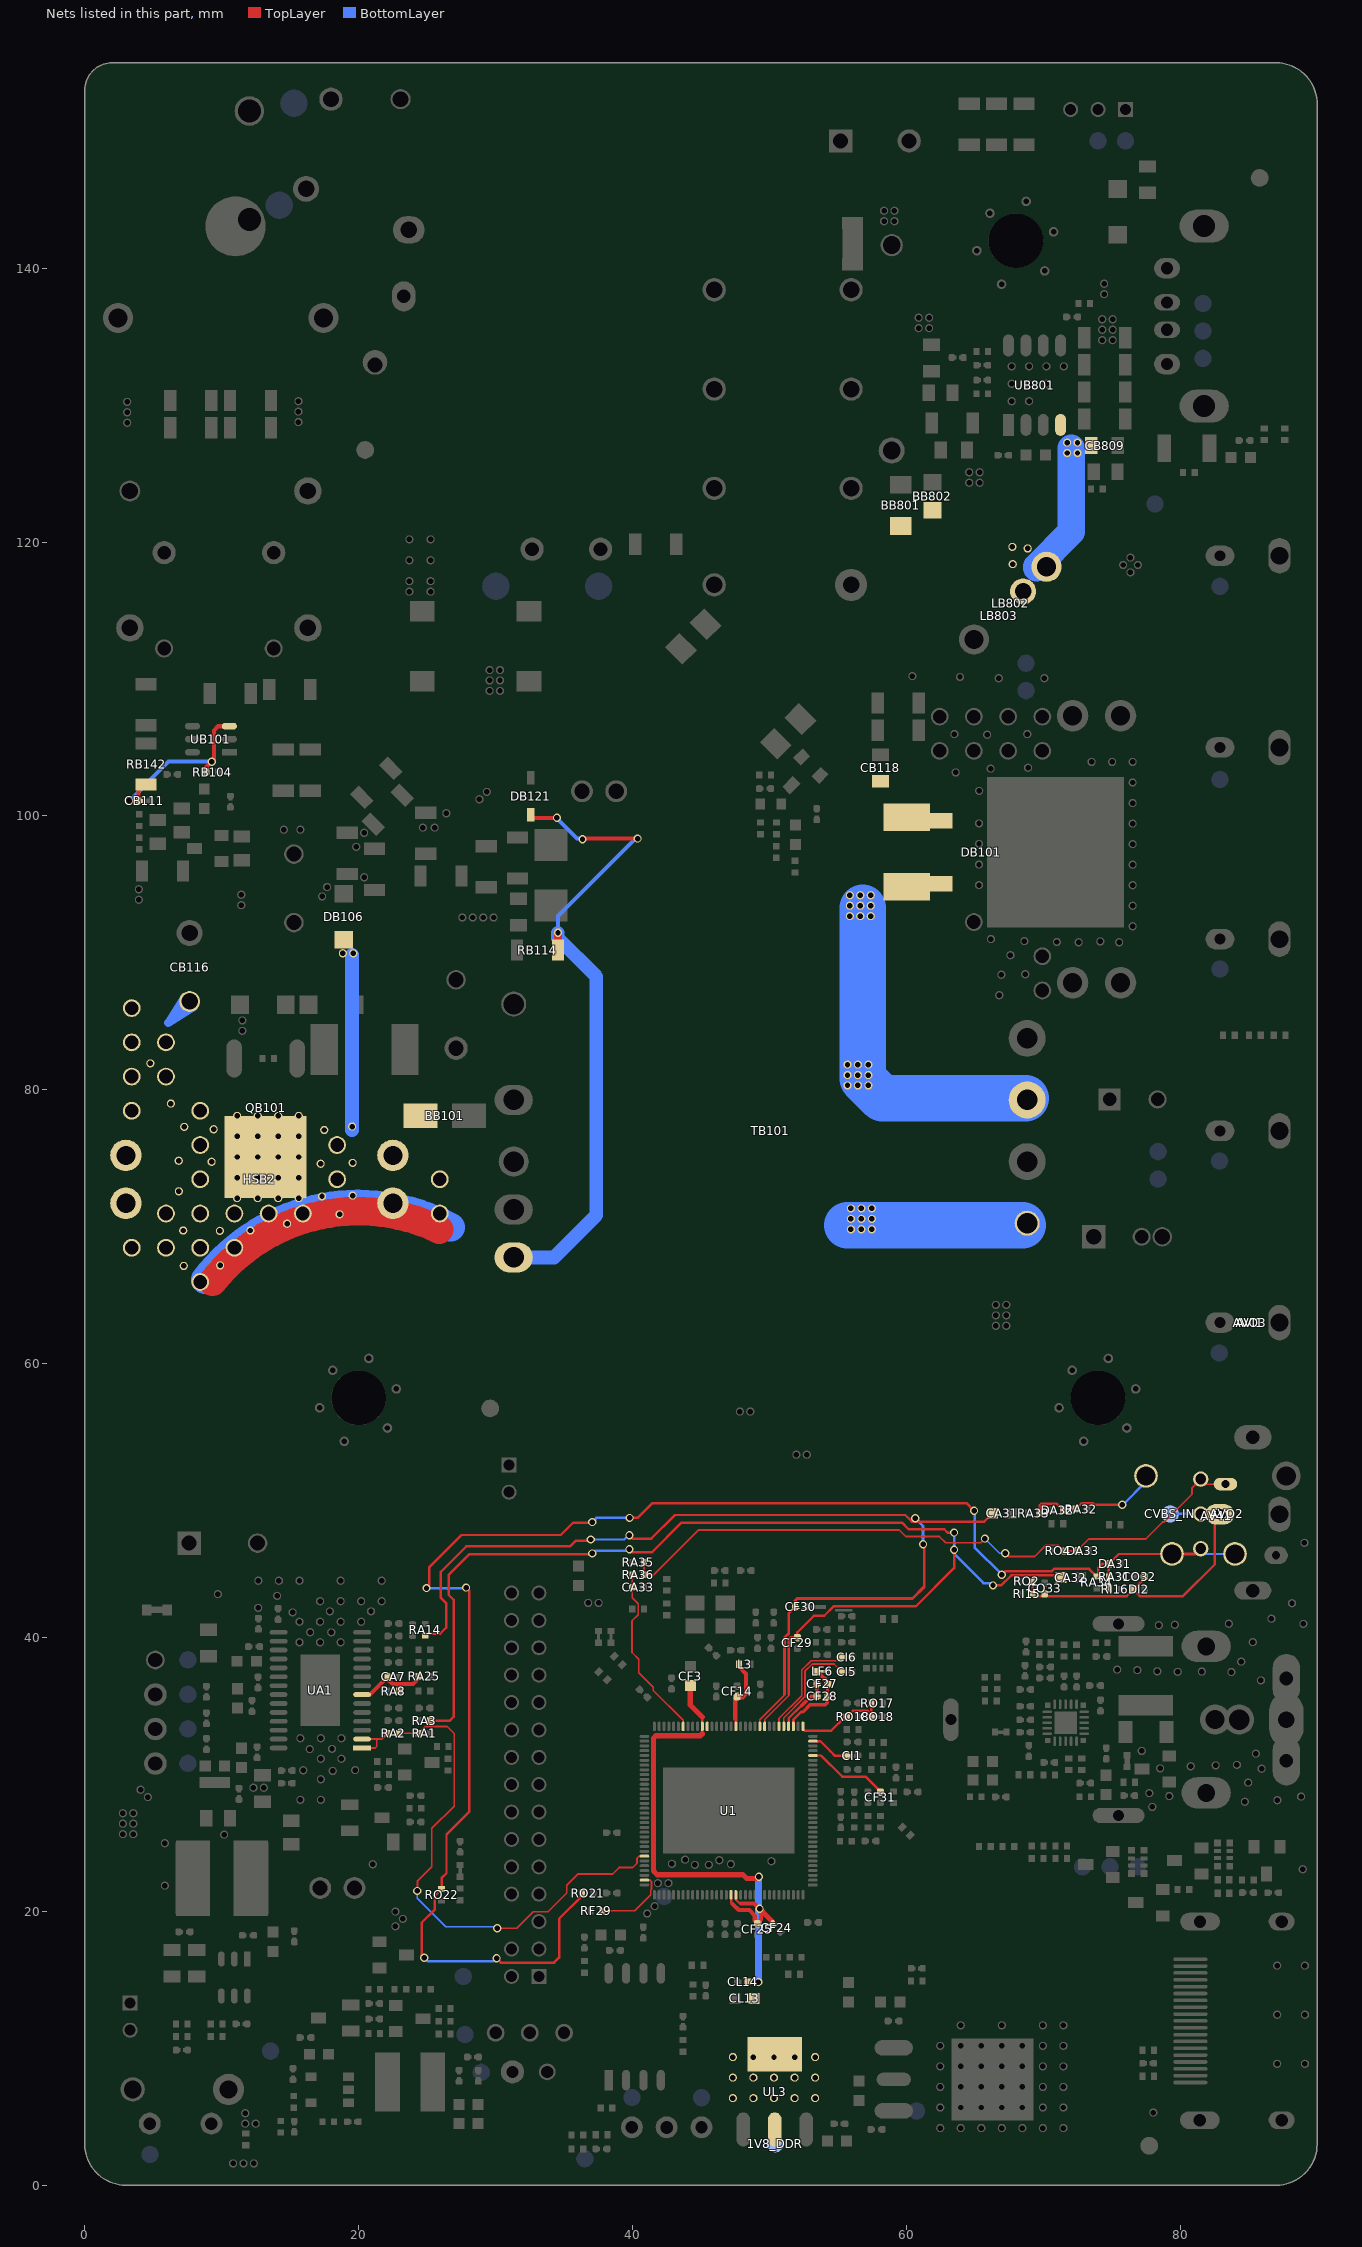
[diagram p0: the nets of this part, all layers, seen from the top]
# Altium PCB MISC116569.PcbDoc (part 7 of 15)
Units mm, origin at the board's own origin, x right, y up, seen from the top; angles counter-clockwise.
Board outline 90 x 155 mm, 2 copper layers (TopLayer, BottomLayer), stack 1.571 mm thick; 527 components, 277 nets, 2450 pads, 649 vias.

## Via types
v1: diameter 0.6, hole 0.4, TopLayer to BottomLayer, tented both sides, 649 vias

## Nets (pads, with @x,y where several pads share a name; then routed paths per layer and width w, separated by ;. In a path a pad name is that pad's centre, name@x,y a point inside that pad or via, vN(x,y) a via of type N, cw(c..) or ccw(c..) an arc to the next point about the centre after c; other vN are vias at no path point) (continued)
12V-COIL: CB118.1 DB101.1 DB101.3 pad.VIA5@55.702,80.315 pad.VIA5@55.702,81.077 pad.VIA5@55.702,81.839 pad.VIA5@55.875,92.685 pad.VIA5@55.875,93.447 pad.VIA5@55.875,94.209 pad.VIA5@55.956,69.812 pad.VIA5@55.956,70.574 pad.VIA5@55.956,71.336 pad.VIA5@56.464,80.315 pad.VIA5@56.464,81.077 pad.VIA5@56.464,81.839 pad.VIA5@56.637,92.685 pad.VIA5@56.637,93.447 pad.VIA5@56.637,94.209 pad.VIA5@56.718,69.812 pad.VIA5@56.718,70.574 pad.VIA5@56.718,71.336 pad.VIA5@57.48,69.812 pad.VIA5@57.48,70.574 pad.VIA5@57.48,71.336 pad.VIA5@57.226,80.315 pad.VIA5@57.226,81.077 pad.VIA5@57.226,81.839 pad.VIA5@57.399,92.685 pad.VIA5@57.399,93.447 pad.VIA5@57.399,94.209 TB101.7 TB101.9 | length 43.5
  BottomLayer w3.4: 55.696,70.11 65.303,70.11 ; pad.VIA5@56.815,93.294 56.815,80.797 58.237,79.375 TB101.9@68.704,79.375 ; 59.544,70.11 65.303,70.11 ; TB101.7@68.504,70.11 65.303,70.11
12V_OVP: DB121.A RB114.2 TB101.6 | length 48
  TopLayer w0.3: DB121.A@32.563,100.089 32.791,99.86 v1@34.442,99.86 ; v1@36.322,98.349 v1(40.373,98.349)
  TopLayer w0.6: RB114.2@34.56,90.208 v1(34.56,91.468)
  BottomLayer w0.3: v1@34.531,99.771 35.954,98.349 v1@36.322,98.349 ; v1(34.56,91.468) 34.56,92.687 v1@40.221,98.349
  BottomLayer w1: TB101.6@31.323,67.756 34.262,67.756 37.363,70.858 37.363,88.265 34.544,91.084 v1@34.544,91.453
  other v1: 36.347,98.298 34.48,99.86
+1.8V_DDR: 1V8_DDR.1 CF3.2 CF24.1 CF25.1 CL13.2 CL14.2@48.306,14.861 CL14.2@48.481,14.861 pad.VIA5@47.334,6.361 pad.VIA5@47.334,7.861 pad.VIA5@47.334,9.361 pad.VIA5@48.834,6.361 pad.VIA5@48.834,7.861 pad.VIA5@48.834,9.361 pad.VIA5@50.334,6.361 pad.VIA5@50.334,7.861 pad.VIA5@50.334,9.361 pad.VIA5@51.834,6.361 pad.VIA5@51.834,7.861 pad.VIA5@51.834,9.361 pad.VIA5@53.334,6.361 pad.VIA5@53.334,7.861 pad.VIA5@53.334,9.361 U1.54 U1.113 U1.114 UL3.2 UL3.4 | length 43.2
  TopLayer w0.178: U1.113@47.199,21.207 47.199,20.652 47.313,20.538 ; U1.114@47.55,21.206 47.573,21.182 47.573,20.832 47.828,20.576
  TopLayer w0.203: 44.885,34.415 45.099,34.201 U1.54@45.099,33.508 45.1,32.963
  TopLayer w0.305: 47.313,20.538 47.757,20.094 48.534,20.094 48.923,19.706 48.923,19.323 CF25.1@49.112,19.133 49.378,19.398 49.378,20.089 v1(49.284,20.183) 48.89,20.576 47.913,20.576
  TopLayer w0.381: CF3.2@44.221,36.479 44.221,35.079 45.099,34.201 ; 45.1,32.963 44.969,32.832 41.727,32.832 41.541,32.645 41.541,22.938 41.801,22.677 47.112,22.677 ; 47.616,22.677 47.112,22.677 ; v1(49.233,22.52) 49.121,22.407 48.339,22.407 48.07,22.677 47.112,22.677 ; v1@49.378,20.089 49.751,19.716 ; 50.027,19.44 49.751,19.716 ; CF24.1@50.224,19.092 50.224,19.242 49.751,19.716
  TopLayer w0.508: UL3.4@49.804,8.881 UL3.4@50.478,9.554
  BottomLayer w0.381: v1@49.208,22.342 49.233,22.367 v1(49.233,22.52)
  BottomLayer w0.508: v1@49.208,14.849 v1@49.208,22.342
  other v1: 49.195,14.836
AMP_L_OUT_IC: CA32.2 CF29.1 RA3.1 U1.41 | length 83.9
  TopLayer w0.127: U1.41@49.649,33.508 49.649,34.015 51.425,35.791 51.425,35.863
  TopLayer w0.178: RA3.1@25.229,33.929 26.659,33.929 26.948,34.217 26.948,42.741 26.568,43.121 26.568,44.566 28.093,46.091 v1@36.993,46.091 ; 39.987,46.23 41.43,46.23 43.589,48.389 59.686,48.389 60.168,47.907 62.771,47.907 63.012,47.666 v1(63.482,47.666) ; 51.425,35.863 51.425,39.871 51.584,40.03 CF29.1@52.04,40.03 52.04,40.379 53.252,41.591 54.004,41.591 54.69,42.277 60.687,42.277 63.482,45.072 v1(63.482,46.408) ; v1(66.327,43.805) 66.923,43.805 67.666,44.548 70.88,44.548 CA32.2@71.295,44.133
  BottomLayer w0.178: v1@37.274,46.347 v1@39.672,46.347 ; v1(63.482,47.666) v1(63.482,46.408) 63.482,46.121 65.629,43.975 v1@66.157,43.975
  other v1: 37.063,46.136 39.771,46.446
AMP_MUTE_OUT: RA2.1 UA1.1 UA1.2 | length 3.7
  TopLayer w0.127: UA1.1@20.254,31.929 21.218,31.929 21.331,32.042 21.331,32.579 ; UA1.2@20.254,32.579 21.331,32.579 ; RA2.1@22.114,33.011 21.682,32.579 21.331,32.579
AMP_MUTE_OUT_IC: RA1.1 RA2.2 U1.90 | length 37.7
  TopLayer w0.127: RA2.2@22.964,33.011 RA1.1@24.379,33.011 24.871,33.503 26.462,33.503 26.973,32.991 26.973,27.681 25.348,26.056 25.348,23.265 24.29,22.207 v1@24.29,21.5 ; v1(30.119,18.76) 30.124,18.765 31.559,18.765 32.761,19.967 33.827,19.967 35.197,21.337 35.197,21.912 36.008,22.723 38.543,22.723 39.021,23.201 40.013,23.201 40.33,23.517 40.33,23.878 40.484,24.032 U1.90@40.873,24.032 U1.90@40.925,24.032
  BottomLayer w0.127: v1(24.285,21.495) 24.285,20.958 26.36,18.883 v1@29.997,18.883
AMP_R_OUT_IC: CA31.2 CF30.1 RA14.1 U1.42 | length 74.4
  TopLayer w0.127: U1.42@49.299,33.508 49.299,33.988 51.13,35.819
  TopLayer w0.178: RA14.1@24.862,40.145 24.998,40.281 25.955,40.281 26.389,40.715 26.389,42.51 26.01,42.889 26.01,44.798 27.861,46.65 35.446,46.65 35.873,47.077 36.871,47.077 v1(36.952,47.158) ; v1(39.771,47.462) 40.018,47.216 41.362,47.216 43.094,48.948 59.917,48.948 60.4,48.466 ; v1(60.65,48.716) 60.4,48.466 ; CA31.2@66.294,49.075 65.684,48.466 60.4,48.466
  TopLayer w0.203: 51.103,35.846 51.108,35.851 51.108,40.003 51.417,40.312 51.417,41.778 CF30.1@51.869,42.23 51.869,42.681 52.036,42.848 60.45,42.848 61.306,43.704 61.306,46.731 v1(61.222,46.815)
  BottomLayer w0.178: v1(36.952,47.158) 39.394,47.158 39.699,47.462 v1(39.771,47.462)
  BottomLayer w0.203: v1(60.65,48.716) 61.222,48.145 v1(61.222,46.815)
AU_CTRL_IC: U1.53
AUVAG: CF27.2@53.443,36.614 CF27.2@53.618,36.614 CF28.2@53.443,35.7 CF28.2@53.618,35.7 U1.36 | length 4.2
  TopLayer w0.178: U1.36@51.399,33.508 51.399,34.099 52.304,35.004
  TopLayer w0.254: 52.344,35.004 53.04,35.7 CF28.2@53.443,35.7 CF27.2@53.443,36.614
AUVRM: CF27.1 CF28.1 LF6.2 LF6.3 U1.35 | length 6.2
  TopLayer w0.203: U1.35@51.749,33.508 51.749,34 52.315,34.566 52.445,34.566 52.502,34.623
  TopLayer w0.254: 52.502,34.623 52.96,35.081 54.067,35.081 54.241,35.254 CF27.1@54.241,36.614 ; LF6.2@53.442,37.519 53.494,37.519 53.973,37.04 54.019,37.04 54.292,36.767 CF27.1@54.292,36.614
AV1_CVBS_IN_IC: CI1.1 U1.31 | length 3.1
  TopLayer w0.178: U1.31@53.175,32.432 53.709,32.432 54.44,31.702 54.787,31.355 55.619,31.355 CI1.1@55.794,31.355
AV1_L_IN_IC: CI5.1 U1.37 | length 7.8
  TopLayer w0.127: U1.37@51.049,33.508 51.049,34.121 52.59,35.662 52.59,37.527 53.124,38.062 54.716,38.062 55.221,37.556 CI5.1@55.324,37.556
AV1_R_IN_IC: CI6.1 U1.38 | length 8.1
  TopLayer w0.127: U1.38@50.699,33.508 50.699,34.095 52.361,35.757 52.361,37.622 53.042,38.303 54.952,38.303 CI6.1@55.221,38.572
AVCC: CA7.2@22.114,37.145 CA7.2@22.289,37.145 RA8.1 RA25.1 UA1.7 | length 5.7
  TopLayer w0.305: UA1.7@20.204,35.829 UA1.7@20.254,35.829 20.826,35.829 20.976,35.979 CA7.2@22.114,37.118 ; CA7.2@22.114,37.145 CA7.2@22.114,37.118 ; RA8.1@22.964,36.087 22.964,36.525 ; RA25.1@24.379,37.014 23.959,36.594 22.469,36.594 22.114,36.949 CA7.2@22.114,37.118
AVDD_DMPLL: CF14.2@47.638,35.641 CF14.2@47.638,35.816 L3.2 U1.47 | length 5.4
  TopLayer w0.203: U1.47@47.55,33.507 47.55,34.064
  TopLayer w0.305: 47.499,34.064 47.499,35.502 CF14.2@47.638,35.641 48.067,35.641 48.288,35.862 48.288,37.347 47.728,37.907 L3.2@47.728,38.052
BRI_ADJ: RF29.1 U1.95 | length 5.6
  TopLayer w0.127: RF29.1@37.789,20.03 37.8,20.041 40.153,20.041 41.324,21.211 41.324,21.56 41.389,21.625 41.389,22.172 41.279,22.282 U1.95@40.873,22.282
BRO: CB111.1 RB104.1 RB142.1 UB101.3 | length 14.4
  TopLayer w0.3: v1(3.251,101.092) 3.257,101.098 CB111.1@3.935,101.098 3.935,102.214 4.011,102.291 RB142.1@4.478,102.291 ; RB104.1@8.871,103.2 8.871,103.566 v1(9.267,103.962) 9.423,104.118 9.423,106.236 9.738,106.55 UB101.3@10.558,106.55
  BottomLayer w0.3: v1@3.257,101.098 v1(3.251,101.092) 6.121,103.962 v1@9.414,103.962 ; v1@9.119,103.962 v1(9.267,103.962)
CVBS_IN: AVI1.1 AVO2.2 AVO3.1 CO32.2@77.249,44.452 CO32.2@77.424,44.452 CO33.2@70.104,43.161 CO33.2@70.104,43.336 CVBS_IN.1 DI2.K RI15.1 RO2.2 | length 23.2
  TopLayer w0.178: RO2.2@69.215,44.107 69.215,43.199 69.394,43.019 71.463,43.019 72.022,43.019 72.936,43.019 ; 72.728,43.019 72.936,43.019 ; DI2.K@76.563,43.487 76.096,43.019 72.936,43.019 ; CO32.2@77.424,44.452 77.424,44.335 76.601,43.513 DI2.K@76.563,43.513 77.057,43.019 80.196,43.019 82.529,45.352 82.529,48.629 AVO3.1@82.9,49
  BottomLayer w0.178: CVBS_IN.1@79.268,49.024 AVO2.2@81.5,49.025
CVBS_OUT_IC: CO18.2@57.443,34.194 CO18.2@57.618,34.194 RO17.1 RO18.2 U1.33 | length 7.1
  TopLayer w0.178: U1.33@52.449,33.508 52.449,33.324 52.573,33.2 54.516,33.2 55.51,34.194 RO18.2@55.646,34.194 56.086,34.635 57.177,34.635 CO18.2@57.443,34.369 ; CO18.2@57.443,34.194 CO18.2@57.443,34.369 ; RO17.1@57.443,35.204 CO18.2@57.443,34.369 ; CO18.2@57.53,34.282 CO18.2@57.618,34.194
D_QB101: BB101.1 CB116.2 DB106.A HSB2.1 HSB2.2 HSB2.3 HSB2.4 pad.VIA5@3.427,68.463 pad.VIA5@3.427,78.463 pad.VIA5@3.427,80.963 pad.VIA5@3.427,83.463 pad.VIA5@3.427,85.963 pad.VIA5@4.788,81.928 pad.VIA5@5.927,68.463 pad.VIA5@5.927,70.963 pad.VIA5@5.927,80.963 pad.VIA5@5.927,83.463 pad.VIA5@6.286,78.994 pad.VIA5@6.858,74.816 pad.VIA5@6.871,72.583 pad.VIA5@7.188,69.723 pad.VIA5@7.226,67.132 pad.VIA5@7.264,77.292 pad.VIA5@8.427,65.964 pad.VIA5@8.427,68.463 pad.VIA5@8.427,70.963 pad.VIA5@8.427,73.464 pad.VIA5@8.427,75.964 pad.VIA5@8.427,78.464 pad.VIA5@9.258,74.739 pad.VIA5@9.411,77.114 pad.VIA5@9.868,69.698 pad.VIA5@9.881,67.17 pad.VIA5@10.927,68.464 pad.VIA5@10.927,70.964 pad.VIA5@11.126,72.091 pad.VIA5@11.126,73.591 pad.VIA5@11.126,75.091 pad.VIA5@11.126,76.591 pad.VIA5@11.126,78.091 pad.VIA5@12.09,69.723 pad.VIA5@12.626,72.091 pad.VIA5@12.626,73.591 pad.VIA5@12.626,75.091 pad.VIA5@12.626,76.591 pad.VIA5@12.626,78.091 pad.VIA5@13.427,70.964 pad.VIA5@14.77,70.218 pad.VIA5@14.126,72.091 pad.VIA5@14.126,73.591 pad.VIA5@14.126,75.091 pad.VIA5@14.126,76.591 pad.VIA5@14.126,78.091 pad.VIA5@15.626,72.091 pad.VIA5@15.626,73.591 pad.VIA5@15.626,75.091 pad.VIA5@15.626,76.591 pad.VIA5@15.626,78.091 pad.VIA5@15.927,70.964 pad.VIA5@17.221,74.6 pad.VIA5@17.323,72.212 pad.VIA5@17.488,77.064 pad.VIA5@18.427,73.464 pad.VIA5@18.427,75.964 pad.VIA5@18.605,70.904 pad.VIA5@18.848,89.967 pad.VIA5@19.52,77.318 pad.VIA5@19.61,89.967 pad.VIA5@19.558,72.276 pad.VIA5@19.558,74.663 pad.VIA5@25.927,70.964 pad.VIA5@25.927,73.463 QB101.D | length 51.5
  TopLayer w1: DB106.A@18.898,90.96 DB106.A@18.922,90.96
  TopLayer w2.1: 9.32,65.98 cw(c20,57.502) 25.882,69.804
  BottomLayer w1: pad.VIA5@19.52,77.056 19.52,89.852 19.52,89.432
  BottomLayer w2.1: pad.VIA5@8.802,66.153 cw(c20,57.502) 26.723,69.954
DRIM: BB801.1 BB802.1 CB809.2 LB802.2 LB803.2 pad.VIA5@67.742,119.647 pad.VIA5@67.767,118.389 pad.VIA5@68.859,119.532 pad.VIA5@71.737,126.505 pad.VIA5@71.737,127.267 pad.VIA5@72.499,126.505 pad.VIA5@72.499,127.267 UB801.4 | length 9.8
  BottomLayer w2: LB802.2@69.507,118.115 69.507,118.197 72.055,120.744 72.055,126.858
EPH_DET_IN/GND: AV41.6 AVO2.3 DA33.K RA35.1 RA36.2 RO4.2 | length 50.6
  TopLayer w0.127: RA35.1@40.844,45.494 40.844,44.585 RA36.2@40.838,44.579 41.557,44.579 44.833,47.856 59.465,47.856 59.947,47.373 62.412,47.373 62.869,46.916 65.423,46.916 v1(65.733,47.226) ; v1(67.228,46.156) 67.465,45.919 69.365,45.919 70.181,46.734 71.087,46.734 RO4.2@71.502,46.319 DA33.K@72.455,46.319 73.332,47.196 74.79,47.196 ; 73.535,47.196 74.79,47.196 ; AVO2.3@81.173,51.238 AVO2.3@81.5,51.565 ; AV41.6@83.3,51.2 81.865,51.2 AVO2.3@81.5,51.565 ; 74.79,47.196 77.476,47.196 78.707,48.428 78.815,48.428 80.865,50.478 80.865,50.931 AVO2.3@81.5,51.565
  BottomLayer w0.127: v1(65.733,47.226) 66.804,46.156 v1(67.228,46.156)
EPH_DET_IN_IC: CA33.2@39.985,43.665 CA33.2@40.16,43.665 RA36.1 U1.58 | length 13.1
  TopLayer w0.127: RA36.1@39.988,44.579 39.988,42.902 40.419,42.471 40.419,41.67 39.967,41.217 39.967,38.902 40.464,38.406 40.464,37.415 41.523,36.356 41.523,36.127 43.699,33.951 U1.58@43.699,33.508 U1.58@43.649,33.558
EPH_LOUT/COAX: AV41.4 AV41.5 AVO2.1 DA31.K RA31.2 RA34.2 RI16.2 RO21.1 RO22.2 | length 118.2
  TopLayer w0.178: v1@24.612,16.781 24.612,19.185 25.563,20.135 25.563,21.141 RO22.2@26.056,21.634 26.056,22.428 26.415,22.787 26.415,25.614 28.066,27.264 28.066,43.431 ; 25.171,43.828 25.171,45.145 27.514,47.488 34.758,47.488 35.655,48.385 v1@37.059,48.385 ; v1(30.069,16.576) 30.386,16.258 34.276,16.258 34.645,16.627 34.645,19.455 36.273,21.084 RO21.1@36.273,21.339 ; v1(39.789,48.73) 40.378,48.73 41.458,49.809 64.389,49.809 v1(64.948,49.251) ; v1@66.972,44.575 v1(66.972,44.588) 67.211,44.827 70.608,44.827 70.786,45.005 73.346,45.005 RA34.2@73.901,44.45 74.028,44.323 74.028,45.087 74.32,45.38 DA31.K@74.792,45.38 ; RI16.2@74.792,43.523 DA31.K@74.792,45.38 ; AV41.5@79.4,46.1 75.513,46.1 DA31.K@74.792,45.38
  TopLayer w0.203: AV41.5@79.4,46.1 81.115,46.1 AVO2.1@81.5,46.485
  BottomLayer w0.178: v1(24.787,16.607) 25.037,16.356 29.849,16.356 v1(30.069,16.576) ; v1(24.955,43.612) v1@27.808,43.612 ; v1@30.113,16.531 v1@30.158,16.576 ; v1(37.059,48.425) 37.363,48.73 v1(39.789,48.73) ; v1@64.989,49.21 64.989,46.571 v1(66.972,44.588) ; AV41.5@79.4,46.1 AV41.4@84,46.1
  other v1: 27.846,43.65
EPH_ROUT: AV41.3 DA32.K RA32.2 RA33.2 | length 9.9
  TopLayer w0.178: RA33.2@69.743,49.088 69.743,49.652 69.873,49.782 70.967,49.782 DA32.K@71.458,49.291 71.545,49.378 RA32.2@72.365,49.378 72.805,49.818 73.622,49.818 73.742,49.698 v1(75.763,49.698)
  BottomLayer w0.178: v1@75.814,49.698 77.5,51.383 AV41.3@77.5,51.8
GIN1N: CF31.1 U1.28 | length 6
  TopLayer w0.178: U1.28@53.175,31.382 53.774,31.382 55.321,29.836 57.026,29.836 CF31.1@58.102,28.759